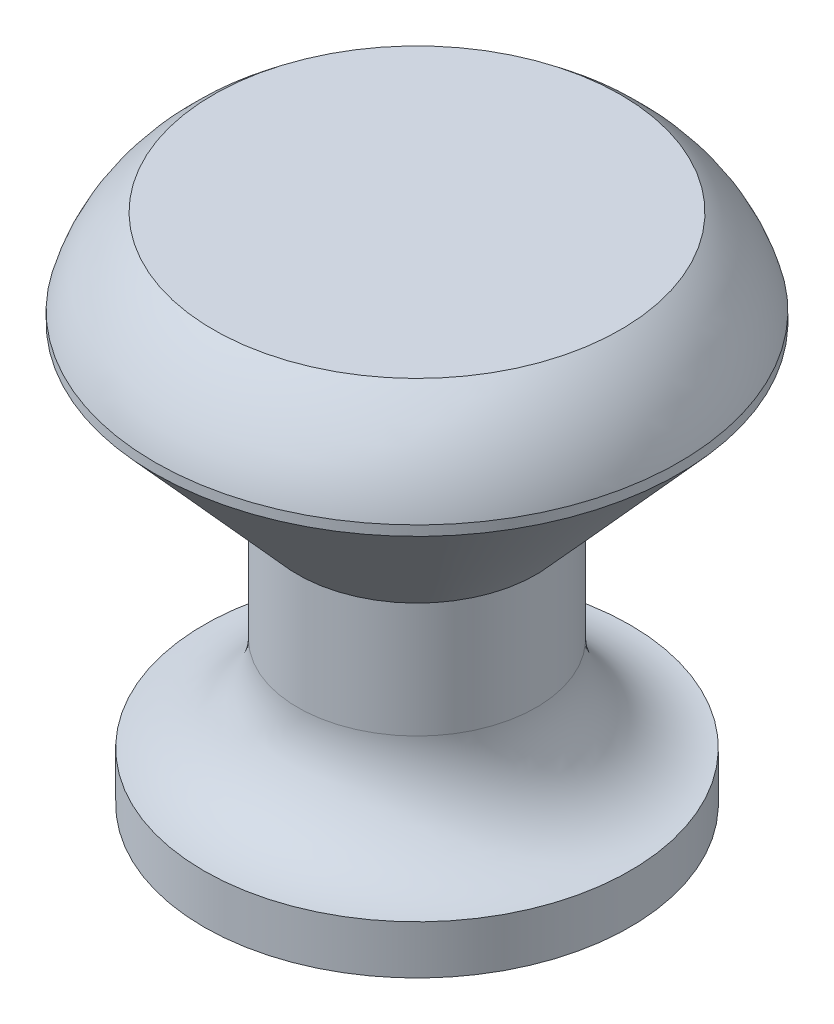
from build123d import *

# Parameters (mm, degrees)
M4_TAPPED_HOLE1_D     = 3.3
M4_TAPPED_HOLE1_DEPTH = 10.1
M4_TAPPED_HOLE1_TIP   = 0.991420021


with BuildPart() as part:
    # Sketch1 → Revolve1 (revolve)
    with BuildSketch(Plane(origin=(0, 0, 0), x_dir=(0, 0, -1), z_dir=(1, 0, 0))):
        with BuildLine():
            Line((0, 0), (10.725, 0))
            Line((10.725, 0), (10.725, 2.45))
            ThreePointArc((10.725, 2.45), (7.382093902, 3.853488302), (6, 7.205296327))
            Line((6, 7.205296327), (6, 13))
            Line((6, 13), (13.200228011, 21))
            Line((13.200228011, 21), (13.200228011, 21.5))
            ThreePointArc((13.200228011, 21.5), (12.098891552, 23.906448602), (10.25, 25.8))
            Line((10.25, 25.8), (0, 25.8))
            Line((0, 25.8), (0, 0))
        make_face()
    revolve(axis=Axis((0, 0, 0), (0, 1, 0)))

    # M4 Tapped Hole1
    with Locations(Plane(origin=(0, 0, 0), x_dir=(-1, 0, 0), z_dir=(0, -1, 0))):
        with Locations((0, 0)):
            Hole(M4_TAPPED_HOLE1_D / 2, depth=M4_TAPPED_HOLE1_DEPTH)
            with Locations((0, 0, -(M4_TAPPED_HOLE1_DEPTH + M4_TAPPED_HOLE1_TIP / 2))):  # 118° drill point
                Cone(0, M4_TAPPED_HOLE1_D / 2, M4_TAPPED_HOLE1_TIP, mode=Mode.SUBTRACT)


solid = part.part
